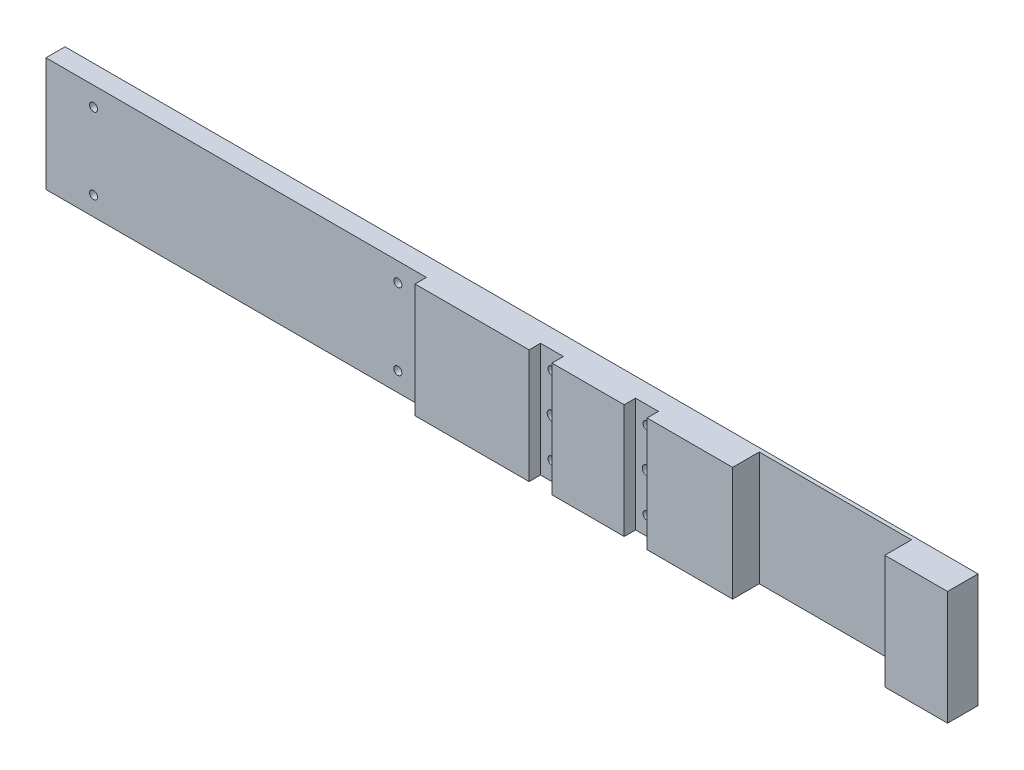
SolidWorks part; units mm, degrees
ref_plane "前视基准面" through (0, 0, 0) normal (0, 0, 1) x (1, 0, 0)
ref_plane "上视基准面" through (0, 0, 0) normal (0, 1, 0) x (1, 0, 0)
ref_plane "右视基准面" through (0, 0, 0) normal (1, 0, 0) x (0, 0, -1)
sketch "草图1" plane through (0, 0, 0) normal (0, 0, 1) x (1, 0, 0)
  line L1 (320.1923, -32.1635) -> (-159.8077, -32.1635)
  line L2 (320.1923, -32.1635) -> (320.1923, 27.8365)
  line L3 (320.1923, 27.8365) -> (-159.8077, 27.8365)
  line L4 (-159.8077, -32.1635) -> (-159.8077, 27.8365)
  dimension "D1" = 60
  dimension "D2" = 480
extrude "凸台-拉伸1" add sketch "草图1" along normal blind 16
sketch "草图2" plane through (0, 0, 16) normal (0, 0, 1) x (1, 0, 0)
  line L0 (-159.8077, -32.1635) -> (320.1923, -32.1635) construction
  line L1 (-159.8077, 27.8365) -> (40.1923, 27.8365)
  line L2 (-159.8077, 27.8365) -> (-159.8077, -32.1635)
  line L3 (-159.8077, -32.1635) -> (40.1923, -32.1635)
  line L4 (40.1923, 27.8365) -> (40.1923, -32.1635)
  dimension "D1" = 200
extrude "切除-拉伸1" cut sketch "草图2" against normal blind 6
sketch "草图3" plane through (0, 0, 16) normal (0, 0, 1) x (1, 0, 0)
  line L0 (100.1923, -32.1635) -> (100.1923, 27.8365)
  line L1 (40.1923, -32.1635) -> (320.1923, -32.1635) construction
  line L2 (320.1923, 27.8365) -> (40.1923, 27.8365) construction
  line L3 (100.1923, 27.8365) -> (112.1923, 27.8365)
  line L4 (112.1923, 27.8365) -> (112.1923, -32.1635)
  line L5 (112.1923, -32.1635) -> (100.1923, -32.1635)
  line L6 (40.1923, -32.1635) -> (40.1923, 27.8365) construction
  line L8 (150.1923, 27.8365) -> (162.1923, 27.8365)
  line L9 (150.1923, 27.8365) -> (150.1923, -32.1635)
  line L10 (150.1923, -32.1635) -> (162.1923, -32.1635)
  line L11 (162.1923, 27.8365) -> (162.1923, -32.1635)
  dimension "D1" = 60
  dimension "D2" = 12
  dimension "D3" = 12
  dimension "D4" = 38
extrude "切除-拉伸2" cut sketch "草图3" against normal blind 6
sketch "草图4" plane through (0, 0, 10) normal (0, 0, 1) x (1, 0, 0)
  line L0 (40.1923, 27.8365) -> (-159.8077, 27.8365) construction
  line L1 (-159.8077, 27.8365) -> (-159.8077, -32.1635) construction
  line L2 (40.1923, -32.1635) -> (40.1923, 27.8365) construction
  line L3 (-159.8077, -32.1635) -> (40.1923, -32.1635) construction
  line L4 (40.1923, -32.1635) -> (40.1923, 27.8365) construction
  line L5 (112.1923, 27.8365) -> (100.1923, 27.8365) construction
  line L6 (112.1923, -32.1635) -> (112.1923, 27.8365) construction
  line L7 (100.1923, -32.1635) -> (112.1923, -32.1635) construction
  line L8 (162.1923, 27.8365) -> (150.1923, 27.8365) construction
  line L9 (150.1923, 27.8365) -> (150.1923, -32.1635) construction
  line L10 (162.1923, -32.1635) -> (162.1923, 27.8365) construction
  line L11 (150.1923, -32.1635) -> (162.1923, -32.1635) construction
  line L12 (112.1923, -32.1635) -> (112.1923, 27.8365) construction
  line L13 (162.1923, -32.1635) -> (162.1923, 27.8365) construction
  circle A0 centre (-134.8077, 17.8365) radius 2.1
  circle A1 centre (-134.8077, -22.1635) radius 2.1
  circle A2 centre (25.1923, 17.8365) radius 2.1
  circle A3 centre (25.1923, -22.1635) radius 2.1
  circle A4 centre (106.1923, 18.3365) radius 2.1
  circle A5 centre (106.1923, -22.6635) radius 2.1
  circle A6 centre (156.1923, 18.3365) radius 2.1
  circle A7 centre (156.1923, -22.6635) radius 2.1
  circle A8 centre (106.1923, -2.1635) radius 2.5
  circle A9 centre (156.1923, -2.1635) radius 2.5
  dimension "D1" = 4.2
  dimension "D2" = 4.2
  dimension "D3" = 4.2
  dimension "D4" = 4.2
  dimension "D13" = 4.2
  dimension "D14" = 4.2
  dimension "D19" = 4.2
  dimension "D21" = 4.2
  dimension "D25" = 5
  dimension "D28" = 5
  dimension "D5" = 10
  dimension "D6" = 25
  dimension "D7" = 10
  dimension "D8" = 15
  dimension "D9" = 10
  dimension "D10" = 25
  dimension "D11" = 10
  dimension "D12" = 15
  dimension "D15" = 9.5
  dimension "D16" = 6
  dimension "D17" = 6
  dimension "D18" = 9.5
  dimension "D20" = 9.5
  dimension "D22" = 6
  dimension "D23" = 6
  dimension "D24" = 9.5
  dimension "D26" = 6
  dimension "D27" = 30
  dimension "D29" = 30
  dimension "D30" = 6
extrude "切除-拉伸3" cut sketch "草图4" against normal through all
sketch "草图5" plane through (0, 0, 16) normal (0, 0, 1) x (1, 0, 0)
  line L0 (207.1923, 27.8365) -> (207.1923, -32.1635)
  line L1 (320.1923, 27.8365) -> (162.1923, 27.8365) construction
  line L2 (162.1923, -32.1635) -> (320.1923, -32.1635) construction
  line L3 (207.1923, -32.1635) -> (287.1923, -32.1635)
  line L4 (287.1923, -32.1635) -> (287.1923, 27.8365)
  line L5 (287.1923, 27.8365) -> (207.1923, 27.8365)
  line L6 (162.1923, -32.1635) -> (162.1923, 27.8365) construction
  dimension "D1" = 80
  dimension "D2" = 45
extrude "切除-拉伸4" cut sketch "草图5" against normal blind 14
